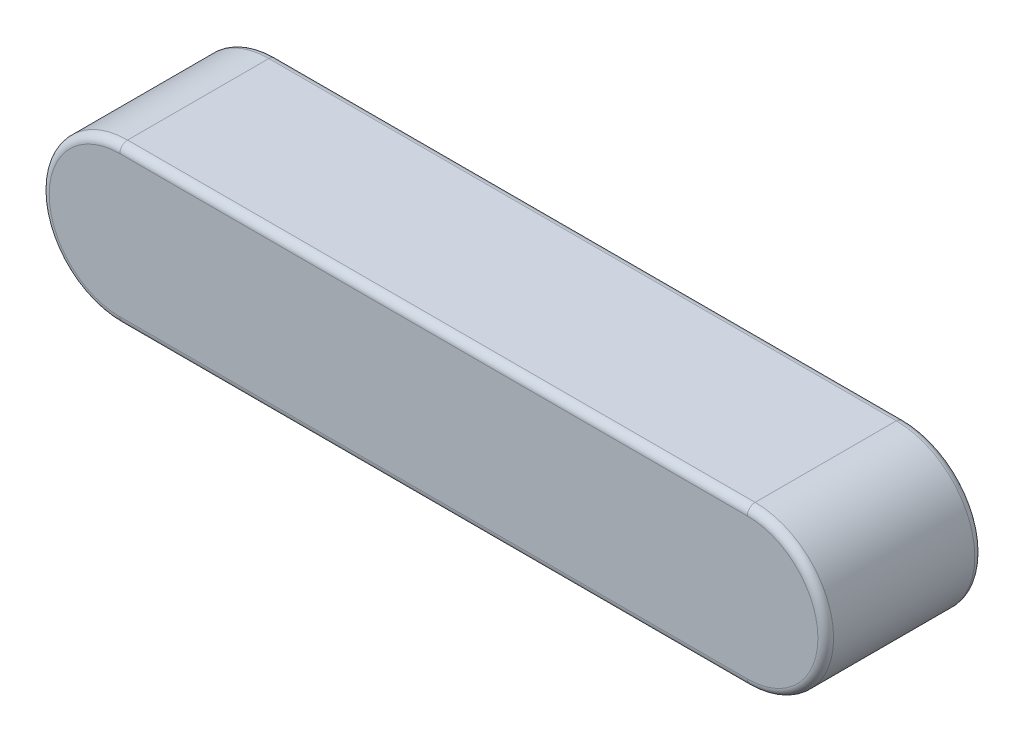
from build123d import *

# Parameters (mm, degrees)
BASE_EXTRUDE_DEPTH = 5
FILLET1_R          = 0.25


with BuildPart() as part:
    # Sketch1 → Base-Extrude (new body)
    with BuildSketch(Plane.XY):
        with BuildLine():
            Line((-10, 2.5), (10, 2.5))
            ThreePointArc((10, 2.5), (12.5, 0), (10, -2.5))
            Line((10, -2.5), (-10, -2.5))
            ThreePointArc((-10, -2.5), (-12.5, 0), (-10, 2.5))
        make_face()
    extrude(amount=BASE_EXTRUDE_DEPTH)

    # Fillet1
    fillet1_edges = [part.edges().sort_by_distance(p)[0] for p in [
        (12.5, 0, 5),
        (0, 2.5, 5),
        (-12.5, 0, 5),
        (0, 2.5, 0),
        (12.5, 0, 0),
        (0, -2.5, 0),
        (-12.5, 0, 0),
        (0, -2.5, 5),
    ]]
    fillet(fillet1_edges, radius=FILLET1_R)


solid = part.part
